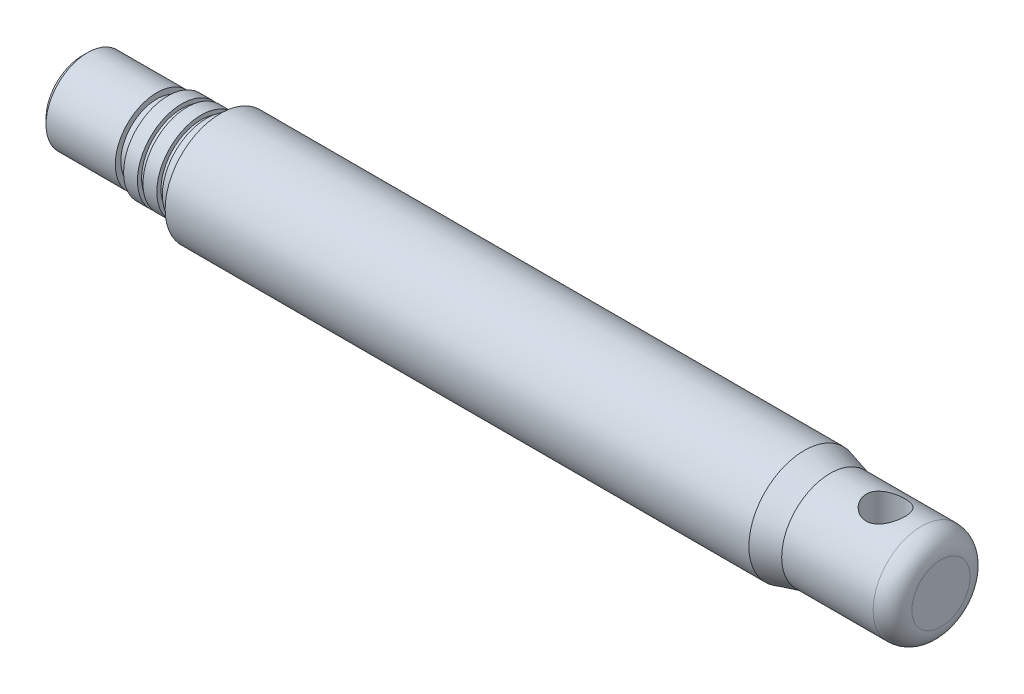
SolidWorks part; units mm, degrees
ref_plane "前视基准面" through (0, 0, 0) normal (0, 0, 1) x (1, 0, 0)
ref_plane "上视基准面" through (0, 0, 0) normal (0, 1, 0) x (1, 0, 0)
ref_plane "右视基准面" through (0, 0, 0) normal (1, 0, 0) x (0, 0, -1)
other "Configuration Table"
sketch "草图1" plane through (0, 0, 0) normal (0, 0, 1) x (1, 0, 0)
  line L0 (0, 0) -> (124.8065, 0) construction
  line L1 (0, 0) -> (0, 15)
  line L2 (0, 15) -> (27, 15)
  line L3 (27, 15) -> (27, 13)
  line L4 (27, 13) -> (31, 13)
  line L5 (31, 13) -> (31, 16)
  line L6 (31, 16) -> (36, 16)
  line L7 (36, 16) -> (36, 14.5)
  line L8 (36, 14.5) -> (38, 14.5)
  line L9 (38, 14.5) -> (38, 16)
  line L10 (38, 16) -> (43, 16)
  line L11 (43, 16) -> (43, 14.5)
  line L12 (43, 14.5) -> (45, 14.5)
  line L13 (45, 14.5) -> (45, 16)
  line L14 (45, 16) -> (50, 16)
  line L15 (50, 16) -> (50, 20)
  line L16 (50, 20) -> (260.6699, 20)
  line L17 (260.6699, 20) -> (270, 17.5)
  line L18 (270, 17.5) -> (310, 17.5)
  line L19 (310, 17.5) -> (310, 0)
  line L20 (124.8065, 0) -> (310, 0) construction
  line L21 (0, 0) -> (310, 0)
  point P13 (27, 14)
  dimension "D1" = 35
  dimension "D2" = 40
  dimension "D3" = 15
  dimension "D4" = 30
  dimension "D5" = 32
  dimension "D6" = 29
  dimension "D7" = 29
  dimension "D8" = 2
  dimension "D9" = 4
  dimension "D10" = 5
  dimension "D11" = 2
  dimension "D12" = 2
  dimension "D13" = 5
  dimension "D14" = 5
  dimension "D15" = 50
  dimension "D16" = 32
  dimension "D17" = 32
  dimension "D18" = 310
  dimension "D19" = 220
revolve "旋转1" add sketch "草图1" angle 360 about L21
cosmetic thread "装饰螺纹线1" parameters "D2"=26.211
sketch "草图2" plane through (0, 0, 0) normal (0, 1, 0) x (1, 0, 0)
  line L0 (310, 0) -> (290, 0) construction
  line L1 (310, -17.5) -> (310, 17.5) construction
  circle A0 centre (290, 0) radius 7
  dimension "D1" = 14
  dimension "D2" = 20
extrude "切除-拉伸1" cut sketch "草图2" against normal through all both and the other way through all
chamfer "倒角1" distance 2 angle 45 1 edges at (0, 0, 15)
fillet "圆角1" radius 7 1 edges at (310, 0, 17.5)
